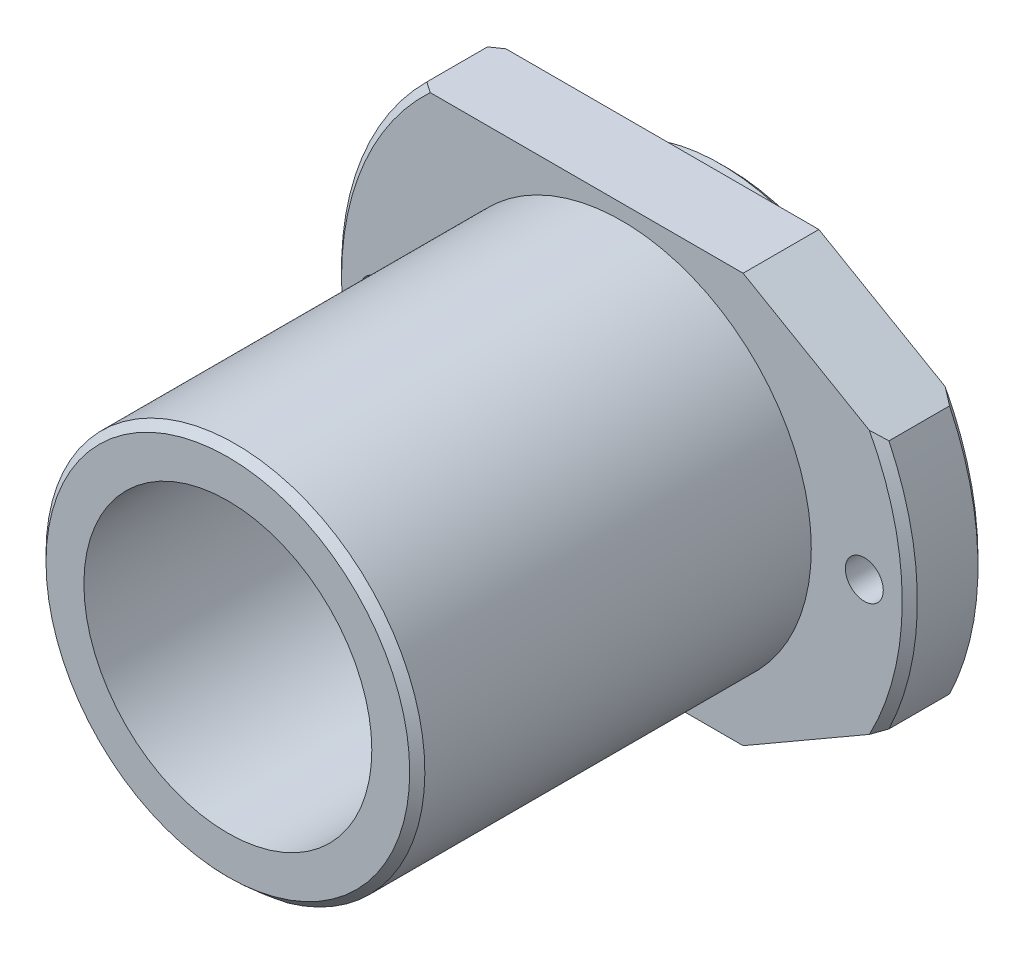
SolidWorks part; units mm, degrees
ref_plane "Front Plane" through (0, 0, 0) normal (0, 0, 1) x (1, 0, 0)
ref_plane "Top Plane" through (0, 0, 0) normal (0, 1, 0) x (1, 0, 0)
ref_plane "Right Plane" through (0, 0, 0) normal (1, 0, 0) x (0, 0, -1)
sketch "Sketch1" plane through (0, 0, 0) normal (0, 0, 1) x (1, 0, 0)
  circle A0 centre (0, 0) radius 12.5
  dimension "D1" = 25
extrude "Boss-Extrude1" add sketch "Sketch1" along normal blind 26
sketch "Sketch2" plane through (0, 0, 0) normal (0, 0, -1) x (-1, 0, 0)
  circle A0 centre (0, 0) radius 19
  dimension "D1" = 38
extrude "Boss-Extrude2" add sketch "Sketch2" along normal blind 5
sketch "Sketch3" plane through (0, 0, -5) normal (0, 0, -1) x (-1, 0, 0)
  circle A0 centre (0, 0) radius 12.5
  circle A1 centre (0, 0) radius 12.5 construction
extrude "Boss-Extrude3" add sketch "Sketch3" along normal blind 2
chamfer "Chamfer1" distance 0.5 angle 45 4 edges at (-19, 0, -5) (12.5, 0, 26) (-12.5, 0, -7) (-19, 0, 0)
sketch "Sketch4" plane through (0, 0, 0) normal (0, 0, 1) x (1, 0, 0)
  line L0 (35.5742, 0) -> (-35.5742, 0) construction
  line L1 (27.9502, -24.8382) -> (-28.8178, -24.8382)
  line L2 (27.9502, -24.8382) -> (27.9502, -13.5)
  line L3 (27.9502, -13.5) -> (-28.8178, -13.5)
  line L4 (-28.8178, -24.8382) -> (-28.8178, -13.5)
  line L5 (27.3305, 13.5) -> (-28.8178, 13.5)
  line L6 (27.3305, 13.5) -> (27.3305, 28.0875)
  line L7 (27.3305, 28.0875) -> (-28.8178, 28.0875)
  line L8 (-28.8178, 13.5) -> (-28.8178, 28.0875)
  dimension "D1" = 27
extrude "Cut-Extrude1" cut sketch "Sketch4" against normal through all
sketch "Sketch5" plane through (0, 0, 26) normal (0, 0, 1) x (1, 0, 0)
  circle A0 centre (0, 0) radius 9.5
  dimension "D1" = 19
extrude "Cut-Extrude2" cut sketch "Sketch5" against normal through all
hole_wizard "M3 Tapped Hole1" positions "Sketch9" profile "Sketch8" tap size "M3" standard "Gb"
sketch "Sketch9" plane through (0, 0, 0) normal (0, 0, 1) x (1, 0, 0)
  line L0 (16, 0) -> (-16, 0) construction
  point P0 (16, 0)
  point P2 (-16, 0)
  dimension "D1" = 32
sketch "Sketch8" plane through (16, 0, 0) normal (1, 0, 0) x (0, -1, 0)
  line L0 (0, 0) -> (0, 8.2511)
  line L1 (0, 8.2511) -> (1.25, 7.5)
  line L2 (1.25, 7.5) -> (1.25, 0)
  line L5 (1.25, 0) -> (0, 0)
  line L10 (0, 8.2511) -> (-1.25, 7.5) construction
  line L11 (0, -6.35) -> (0, 107.95) construction
  dimension "螺纹孔钻头直径" = 2.5
  dimension "螺纹孔钻头深度" = 7.5
  dimension "导头角度" = 118
cosmetic thread "Hole thread 1" parameters "D1"=5, "D2"=3
cosmetic thread "Hole thread 2" parameters "D1"=5, "D2"=3
sketch "Sketch10" plane through (0, 0, 0) normal (0, 0, 1) x (1, 0, 0)
  line L0 (20.899, 6.0527) -> (8, 13.5)
  line L1 (8, 13.5) -> (20.899, 13.5)
  line L2 (20.899, 13.5) -> (20.899, 6.0527)
  line L3 (0, 0) -> (26.9877, 0) construction
  line L4 (-12.6491, 13.5) -> (12.6491, 13.5) construction
  dimension "D1" = 30
  dimension "D2" = 8
extrude "Cut-Extrude3" cut sketch "Sketch10" against normal blind 10
mirror "Mirror1" about plane through (0, 0, 0) normal (0, 1, 0) of "Cut-Extrude3"
sketch "Sketch11" plane through (0, 0, 26) normal (0, 0, 1) x (1, 0, 0)
  line L1 (-24.84, -41.449) -> (35.2953, -41.449)
  line L2 (-24.84, -41.449) -> (-24.84, -12)
  line L3 (-24.84, -12) -> (35.2953, -12)
  line L4 (35.2953, -41.449) -> (35.2953, -12)
  line L5 (-24.84, -41.449) -> (35.2953, -12) construction
  line L6 (-24.84, -12) -> (35.2953, -41.449) construction
  point P0 (5.2277, -26.7245)
  dimension "D1" = 12
extrude "Cut-Extrude4" cut sketch "Sketch11" against normal blind 25
